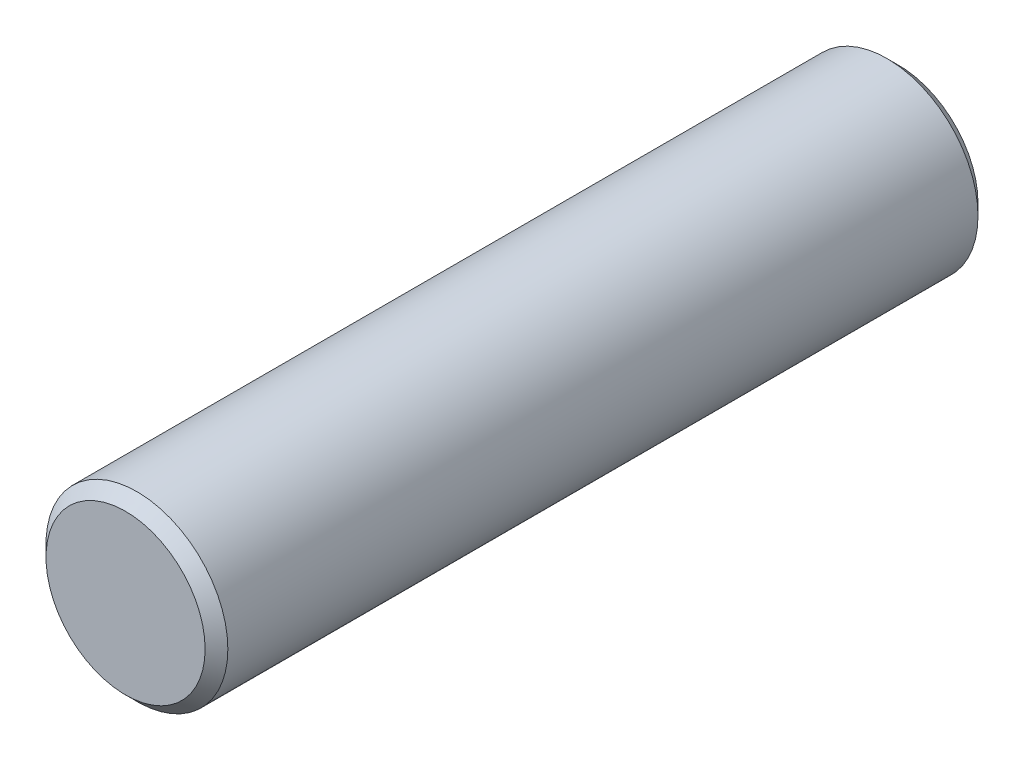
from build123d import *

# Parameters (mm, degrees)
SKETCH1_R           = 4
BOSS_EXTRUDE1_DEPTH = 17
CHAMFER1_SIZE       = 0.5


with BuildPart() as part:
    # Sketch1 → Boss-Extrude1 (new, symmetric)
    with BuildSketch(Plane.XY):
        Circle(SKETCH1_R)
    extrude(amount=BOSS_EXTRUDE1_DEPTH, both=True)

    # Chamfer1
    chamfer1_edges = [part.edges().sort_by_distance(p)[0] for p in [
        (-4, 0, -17),
        (-4, 0, 17),
    ]]
    chamfer(chamfer1_edges, length=CHAMFER1_SIZE)


solid = part.part
